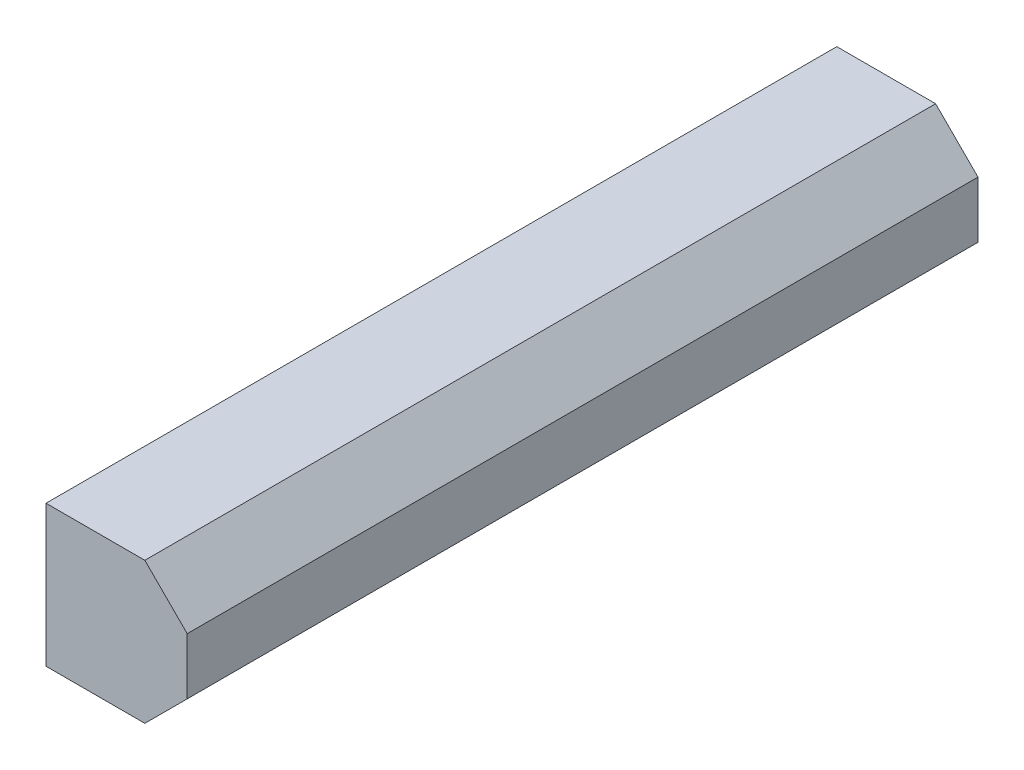
from build123d import *

# Parameters (mm, degrees)
SKETCH1_W           = 280
SKETCH1_H           = 50
BOSS_EXTRUDE1_DEPTH = 25
CHAMFER1_SIZE       = 15


with BuildPart() as part:
    # Sketch1 → Boss-Extrude1 (new, symmetric)
    with BuildSketch(Plane(origin=(0, 0, 0), x_dir=(0, 0, -1), z_dir=(1, 0, 0))):
        Rectangle(SKETCH1_W, SKETCH1_H)
    extrude(amount=BOSS_EXTRUDE1_DEPTH, both=True)

    # Chamfer1
    chamfer1_edges = [part.edges().sort_by_distance(p)[0] for p in [
        (25, 25, 0),
        (25, -25, 0),
    ]]
    chamfer(chamfer1_edges, length=CHAMFER1_SIZE)


solid = part.part
